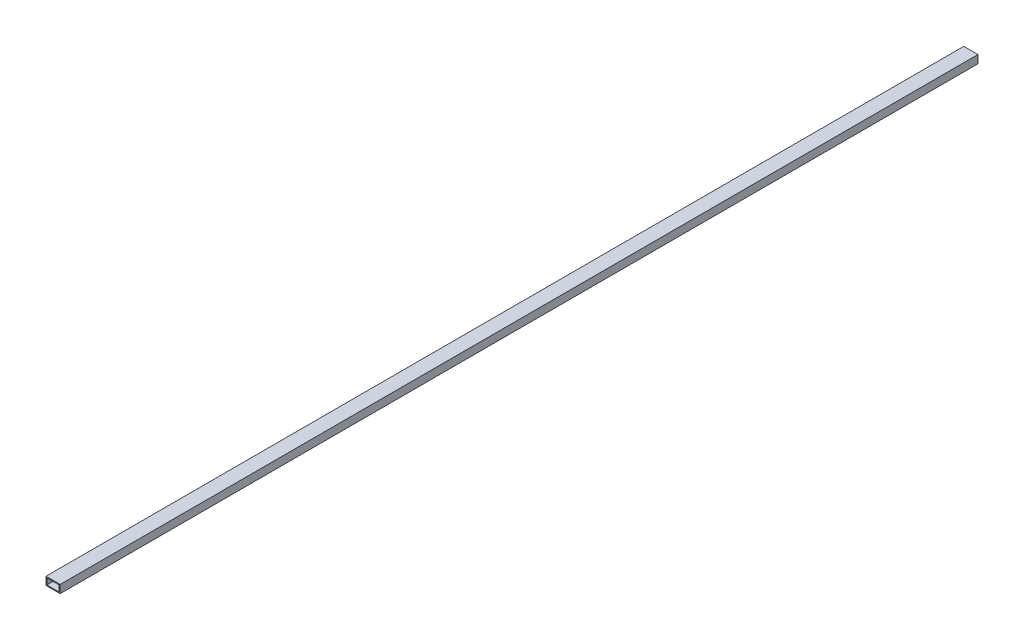
SolidWorks part; units mm, degrees
material "201 annealed stainless steel (SS)"
ref_plane "Front Plane" through (0, 0, 0) normal (0, 0, 1) x (1, 0, 0)
ref_plane "Top Plane" through (0, 0, 0) normal (0, 1, 0) x (1, 0, 0)
ref_plane "Right Plane" through (0, 0, 0) normal (1, 0, 0) x (0, 0, -1)
sketch "Sketch1" plane through (0, 0, 0) normal (0, 0, 1) x (1, 0, 0)
  line L1 (0, 0) -> (20, 0)
  line L2 (0, 0) -> (0, -10)
  line L3 (0, -10) -> (20, -10)
  line L4 (20, 0) -> (20, -10)
  line L5 (0, 0) -> (20, -10) construction
  line L6 (0, -10) -> (20, 0) construction
  point P5 (10, -5)
  dimension "D1" = 10
  dimension "D2" = 20
extrude "Extrude-Thin1" add sketch "Sketch1" along normal blind 1490 thin thin type one direction wall 1.5
